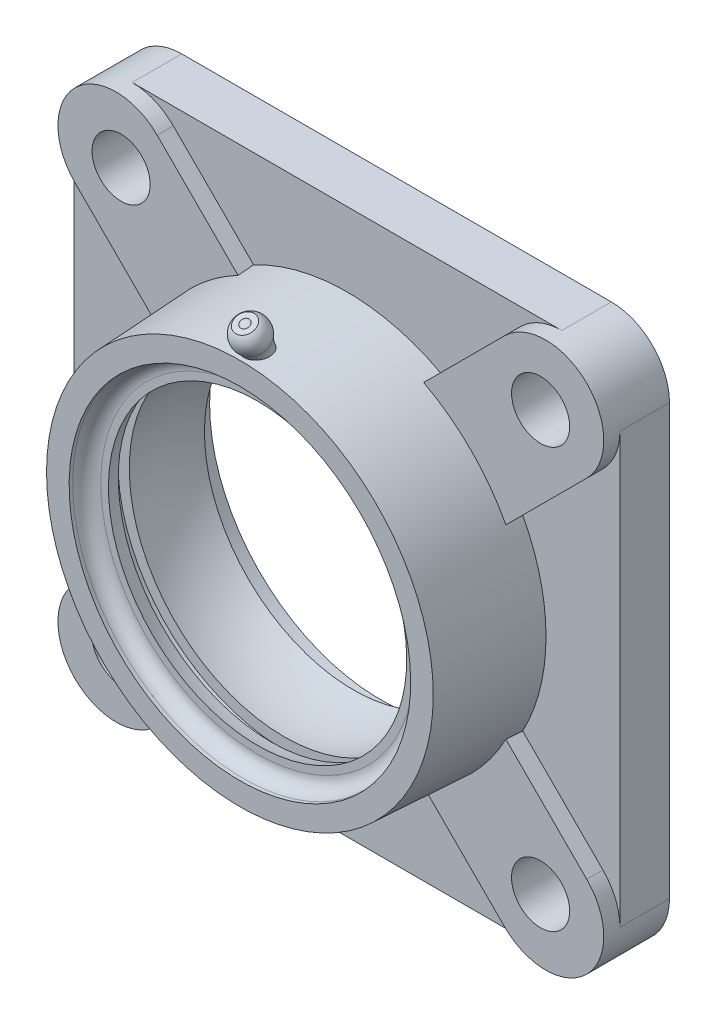
SolidWorks part; units mm, degrees
ref_plane "前视" through (0, 0, 0) normal (0, 0, 1) x (1, 0, 0)
ref_plane "上视" through (0, 0, 0) normal (0, 1, 0) x (1, 0, 0)
ref_plane "右视" through (0, 0, 0) normal (1, 0, 0) x (0, 0, -1)
sketch "尺寸草图" plane through (0, 0, 0) normal (0, 0, 1) x (1, 0, 0)
  line L0 (-92, 0) -> (-30, 0) construction
  line L1 (-54, 54) -> (54, 54)
  line L2 (-54, 54) -> (-54, -54)
  line L3 (-54, -54) -> (54, -54)
  line L4 (54, 54) -> (54, -54)
  circle A0 centre (16, 41.5) radius 5.75
  point P4 (0, 54)
  point P5 (-54, 0)
  point P10 (-72, 0)
  point P11 (-56, 0)
  dimension "N" = 11.5
  dimension "L" = 108
  dimension "J" = 83
  dimension "A" = 38
  dimension "A2" = 20
  dimension "A1" = 16
  dimension "Da" = 62
  dimension "C" = 16
sketch "草图1" plane through (0, 0, 0) normal (0, 0, 1) x (1, 0, 0)
  line L0 (-54, -54) -> (54, -54) construction
  line L1 (54, 54) -> (54, -54) construction
  line L2 (-54, 54) -> (54, 54) construction
  line L3 (-54, 54) -> (-54, -54) construction
  line L4 (-42.5, -54) -> (42.5, -54)
  line L5 (54, 42.5) -> (54, -42.5)
  line L6 (-42.5, 54) -> (42.5, 54)
  line L7 (-54, 42.5) -> (-54, -42.5)
  line L8 (0, 0) -> (54, 0) construction
  line L9 (0, 0) -> (0, 54) construction
  circle A0 centre (-41.5, -41.5) radius 5.75
  circle A1 centre (16, 41.5) radius 5.75 construction
  arc A2 (54, 42.5) -> (42.5, 54) centre (42.5, 42.5) ccw
  arc A3 (-42.5, 54) -> (-54, 42.5) centre (-42.5, 42.5) ccw
  arc A4 (-42.5, -54) -> (-54, -42.5) centre (-42.5, -42.5) cw
  arc A5 (42.5, -54) -> (54, -42.5) centre (42.5, -42.5) ccw
  circle A6 centre (-41.5, 41.5) radius 5.75
  circle A7 centre (41.5, -41.5) radius 5.75
  circle A8 centre (41.5, 41.5) radius 5.75
  dimension "D1" = 11.5
extrude "基体-拉伸" add sketch "草图1" along normal blind 9.8
sketch "草图2" plane through (0, 0, 0) normal (0, 0, 1) x (1, 0, 0)
  line L0 (-50.6317, -34.3683) -> (-18.7635, -2.5)
  line L1 (-18.7635, -2.5) -> (-2.5, -18.7635)
  line L2 (-2.5, -18.7635) -> (-34.3683, -50.6317)
  line L3 (0, 0) -> (0, -54) construction
  line L4 (-42.5, -54) -> (42.5, -54) construction
  line L5 (0, 0) -> (-54, 0) construction
  line L6 (-54, 42.5) -> (-54, -42.5) construction
  line L7 (-18.7635, 2.5) -> (-2.5, 18.7635)
  line L8 (-50.6317, 34.3683) -> (-18.7635, 2.5)
  line L9 (-2.5, 18.7635) -> (-34.3683, 50.6317)
  line L10 (2.5, -18.7635) -> (34.3683, -50.6317)
  line L11 (2.5, 18.7635) -> (34.3683, 50.6317)
  line L12 (18.7635, 2.5) -> (2.5, 18.7635)
  line L13 (18.7635, -2.5) -> (2.5, -18.7635)
  line L14 (50.6317, 34.3683) -> (18.7635, 2.5)
  line L15 (50.6317, -34.3683) -> (18.7635, -2.5)
  arc A0 (-50.6317, -34.3683) -> (-34.3683, -50.6317) centre (-42.5, -42.5) ccw
  arc A1 (-54, -42.5) -> (-42.5, -54) centre (-42.5, -42.5) ccw construction
  arc A2 (-50.6317, 34.3683) -> (-34.3683, 50.6317) centre (-42.5, 42.5) cw
  arc A3 (50.6317, 34.3683) -> (34.3683, 50.6317) centre (42.5, 42.5) ccw
  arc A4 (50.6317, -34.3683) -> (34.3683, -50.6317) centre (42.5, -42.5) cw
  circle A5 centre (41.5, 41.5) radius 5.75 construction
  circle A6 centre (41.5, -41.5) radius 5.75 construction
  circle A7 centre (-41.5, -41.5) radius 5.75 construction
  circle A8 centre (-41.5, 41.5) radius 5.75 construction
  circle A9 centre (41.5, 41.5) radius 5.75
  circle A10 centre (41.5, -41.5) radius 5.75
  circle A11 centre (-41.5, -41.5) radius 5.75
  circle A12 centre (-41.5, 41.5) radius 5.75
  dimension "D1" = 45
  dimension "D2" = 5
extrude "凸台-拉伸1" add sketch "草图2" along normal blind 13
sketch "草图3" plane through (0, 0, 0) normal (0, 0, 1) x (1, 0, 0)
  line L0 (41.5, 41.5) -> (-41.5, -41.5) construction
  line L1 (-41.5, 41.5) -> (41.5, -41.5) construction
  line L3 (-41.5, 41.5) -> (-42.6873, 40.3127) construction
  line L4 (41.5, -41.5) -> (42.8302, -40.1698) construction
  line L5 (-26.7574, 48.125) -> (26.7574, 48.125)
  line L6 (41.5, 41.5) -> (40, 43) construction
  line L7 (-41.5, -41.5) -> (-40, -43) construction
  line L8 (-26.7574, -48.125) -> (26.7574, -48.125)
  line L9 (0, 0) -> (46.4612, 0) construction
  line L10 (-48.125, 26.7574) -> (-48.125, -6.625)
  line L11 (48.125, -26.7574) -> (48.125, 6.625)
  line L12 (0, 0) -> (0, -23.084) construction
  line L13 (-41.5, -26.1386) -> (-41.5, -12.625)
  line L14 (-44.5, -9.625) -> (-45.125, -9.625)
  line L15 (41.5, 26.1386) -> (41.5, 12.625)
  line L16 (44.5, 9.625) -> (45.125, 9.625)
  arc A0 (-29.6007, 44.1681) -> (-44.1681, 29.6007) centre (-40.5, 40.5) cw
  arc A1 (-42.5, 54) -> (-54, 42.5) centre (-42.5, 42.5) ccw construction
  arc A2 (29.6007, -44.1681) -> (44.1681, -29.6007) centre (40.5, -40.5) cw
  arc A3 (42.5, -54) -> (54, -42.5) centre (42.5, -42.5) ccw construction
  arc A4 (-38.9138, -29.1099) -> (-29.6007, -44.1681) centre (-40.5, -40.5) cw
  arc A5 (54, 42.5) -> (42.5, 54) centre (42.5, 42.5) ccw construction
  arc A6 (29.6007, -44.1681) -> (26.7574, -48.125) centre (26.7574, -45.125) cw
  arc A7 (-29.6007, -44.1681) -> (-26.7574, -48.125) centre (-26.7574, -45.125) ccw
  arc A8 (-38.9138, -29.1099) -> (-41.5, -26.1386) centre (-38.5, -26.1386) cw
  arc A9 (-54, -42.5) -> (-42.5, -54) centre (-42.5, -42.5) ccw construction
  arc A10 (29.6007, 44.1681) -> (38.9138, 29.1099) centre (40.5, 40.5) ccw
  arc A12 (44.1681, -29.6007) -> (48.125, -26.7574) centre (45.125, -26.7574) ccw
  arc A13 (48.125, 6.625) -> (45.125, 9.625) centre (45.125, 6.625) ccw
  arc A14 (-41.5, -12.625) -> (-44.5, -9.625) centre (-44.5, -12.625) ccw
  arc A15 (41.5, 12.625) -> (44.5, 9.625) centre (44.5, 12.625) ccw
  arc A16 (-48.125, -6.625) -> (-45.125, -9.625) centre (-45.125, -6.625) ccw
  arc A17 (-44.1681, 29.6007) -> (-48.125, 26.7574) centre (-45.125, 26.7574) ccw
  arc A18 (-29.6007, 44.1681) -> (-26.7574, 48.125) centre (-26.7574, 45.125) cw
  arc A19 (29.6007, 44.1681) -> (26.7574, 48.125) centre (26.7574, 45.125) ccw
  arc A20 (38.9138, 29.1099) -> (41.5, 26.1386) centre (38.5, 26.1386) cw
  point P22 (0, 0)
  point P60 (-41.5, -9.625)
  point P63 (41.5, 9.625)
  dimension "D1" = 3
  dimension "D2" = 9.625
extrude "切除-拉伸3" cut sketch "草图3" along normal blind 3.2
sketch "草图4" plane through (0, 0, 9.8) normal (0, 0, 1) x (1, 0, 0)
  circle A0 centre (0, 0) radius 39.37
  dimension "D1" = 78.74
extrude "凸台-拉伸2" add sketch "草图4" along normal blind 21.2 draft 3
sketch "草图5" plane through (0, 0, 0) normal (1, 0, 0) x (0, 0, -1)
  line L2 (-31, 33.79) -> (-30.29, 33.79)
  line L3 (-27.5, 31) -> (-27.5, 29.5085)
  line L7 (0, 0) -> (-31, 0) construction
  line L8 (-13, 0) -> (-31, 0) construction
  line L9 (-8.5, 29.5085) -> (-8.5, 31)
  line L10 (-24.8333, 32.9728) -> (-22.1667, 32.9728)
  line L11 (-24.8333, 32.9728) -> (-24.8333, 30.2375)
  line L12 (0, 33.79) -> (-5.71, 33.79)
  line L13 (-22.1667, 32.9728) -> (-22.1667, 30.7187)
  line L14 (-31, 33.79) -> (-31, 0)
  line L15 (-31, 0) -> (0, 0)
  line L16 (0, 0) -> (0, 33.79)
  line L17 (0, 42.5) -> (0, 54) construction
  line L18 (-31, 38.259) -> (-31, -38.259) construction
  arc A0 (-27.5, 29.5085) -> (-24.8333, 30.2375) centre (-18, 0) cw
  arc A1 (-30.29, 33.79) -> (-27.5, 31) centre (-30.29, 31) cw
  arc A2 (-22.1667, 30.7187) -> (-8.5, 29.5085) centre (-18, 0) cw
  arc A3 (-5.71, 33.79) -> (-8.5, 31) centre (-5.71, 31) ccw
  point P18 (-18, 31)
  point P19 (-28.3172, 32.9728)
  dimension "D2" = 31
  dimension "D1" = 18
  dimension "D3" = 19
  dimension "D4" = 33.79
  dimension "D5" = 0
  dimension "D6" = 0
revolve "切除-旋转1" cut sketch "草图5" angle 360 about L7
sketch "草图6" plane through (0, 0, 0) normal (1, 0, 0) x (0, 0, -1)
  line L0 (-24.8333, 32.9728) -> (-30.1215, 44.3132) construction
  line L1 (-24.8333, -32.9728) -> (-24.8333, 32.9728) construction
  line L2 (-13, 54) -> (-13, 34.3683) construction
  line L6 (-22.1667, 32.9728) -> (-24.8333, 32.9728) construction
  line L7 (-28.1423, 34.39) -> (-25.9671, 35.4043)
  line L8 (-28.1423, 34.39) -> (-29.2732, 36.8153)
  line L9 (-31.8063, 43.194) -> (-30.8215, 43.6532)
  line L10 (-9.8, 39.37) -> (-31, 38.259) construction
  line L11 (-25.9671, 35.4043) -> (-30.1215, 44.3132)
  line L13 (-30.29, 33.79) -> (-31, 33.79) construction
  arc A0 (-29.2732, 36.8153) -> (-31.1103, 39.3246) centre (-36.5237, 33.4344) ccw
  arc A1 (-31.1103, 39.3246) -> (-31.8063, 43.194) centre (-28.911, 41.7175) cw
  arc A2 (-30.8215, 43.6532) -> (-30.1215, 44.3132) centre (-29.4745, 42.9259) cw
  dimension "D4" = 8
  dimension "D5" = 3.25
  dimension "D8" = 0.66
  dimension "D1" = 25
  dimension "D2" = 2.4
  dimension "D3" = 6
  dimension "D6" = 4
  dimension "D7" = 0.7
  dimension "D9" = 0.6
revolve "凸台-旋转1" add sketch "草图6" angle 360 about L0
